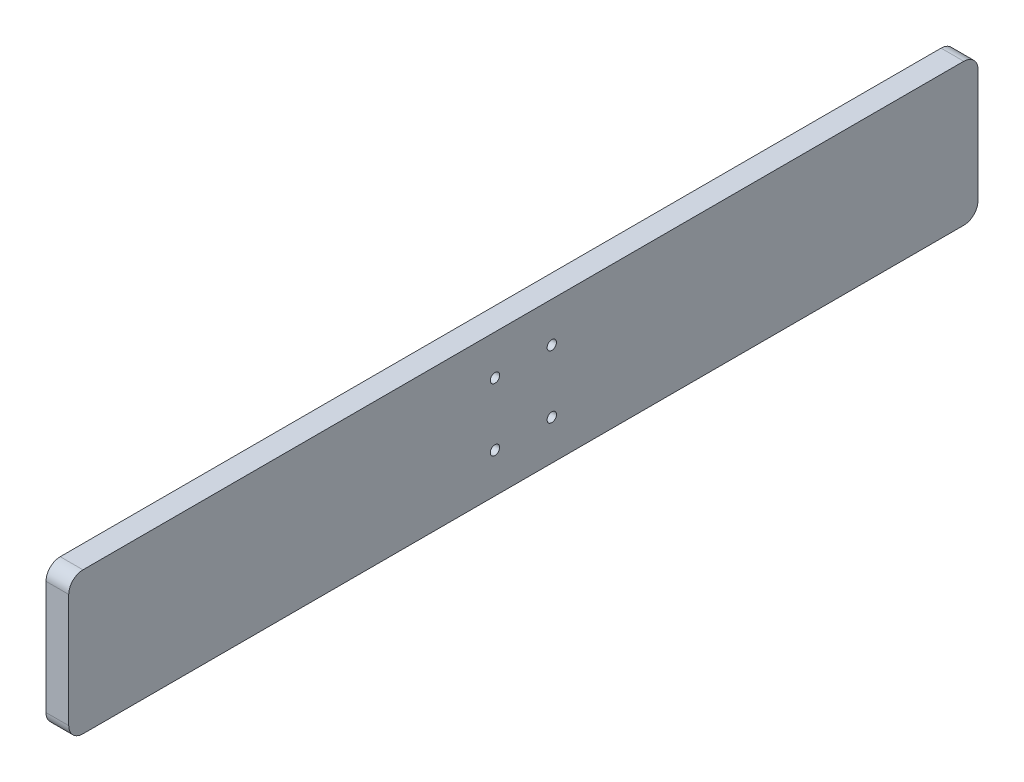
from build123d import *

# Parameters (mm, degrees)
SKETCH_1_W         = 320
SKETCH_1_H         = 50
EXTRUDE_1_DEPTH    = 8
HOLE_WIZARD_M4_1_D = 3.3
FILLET_1_R         = 5


with BuildPart() as part:
    # 草图1 → 凸台-拉伸1 (new body)
    with BuildSketch(Plane(origin=(0, 0, 0), x_dir=(0, 0, -1), z_dir=(1, 0, 0))):
        Rectangle(SKETCH_1_W, SKETCH_1_H)
    extrude(amount=EXTRUDE_1_DEPTH)

    # M4 螺纹孔1 (through all)
    with Locations(Plane.ZY):
        with Locations((-10, -11), (-10, 11), (10, -11), (10, 11)):
            Hole(HOLE_WIZARD_M4_1_D / 2)

    # 圆角1
    fillet_1_edges = [part.edges().sort_by_distance(p)[0] for p in [
        (4, -25, -160),
        (4, -25, 160),
        (4, 25, 160),
        (4, 25, -160),
    ]]
    fillet(fillet_1_edges, radius=FILLET_1_R)


solid = part.part
